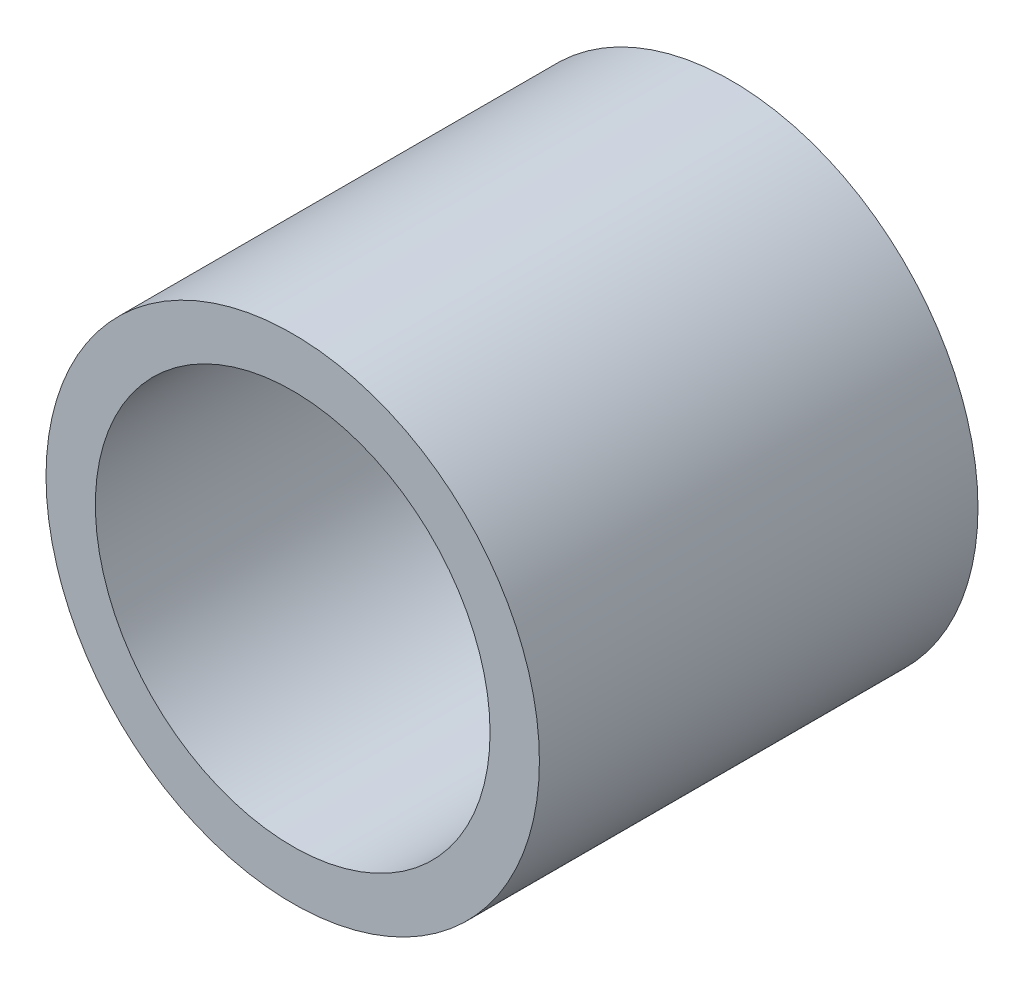
SolidWorks part; units mm, degrees
ref_plane "前视基准面" through (0, 0, 0) normal (0, 0, 1) x (1, 0, 0)
ref_plane "上视基准面" through (0, 0, 0) normal (0, 1, 0) x (1, 0, 0)
ref_plane "右视基准面" through (0, 0, 0) normal (1, 0, 0) x (0, 0, -1)
sketch "草图1" plane through (0, 0, 0) normal (0, 0, 1) x (1, 0, 0)
  circle A0 centre (0, 0) radius 36
  circle A1 centre (0, 0) radius 45
  dimension "D1" = 72
  dimension "D2" = 90
extrude "凸台-拉伸1" add sketch "草图1" along normal mid plane 80
